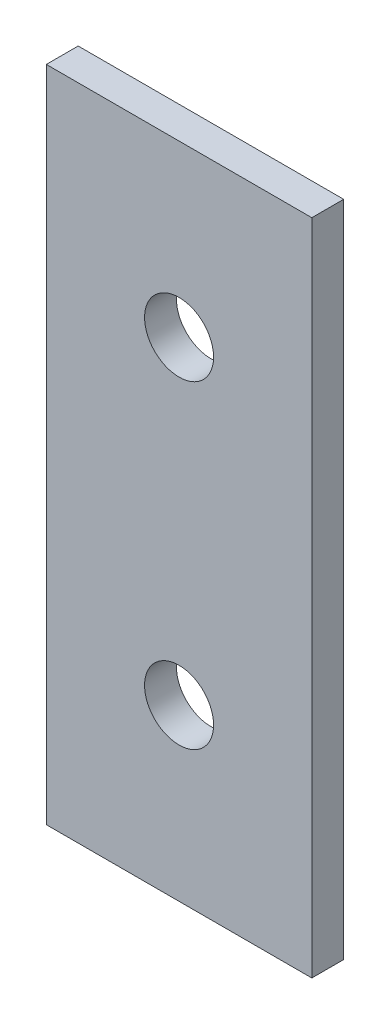
from build123d import *

# Parameters (mm, degrees)
SKETCH1_W          = 50
SKETCH1_H          = 124
EXTRUDE1_DEPTH     = 3
SKETCH2_R          = 6.5
CUT_EXTRUDE1_DEPTH = 22


with BuildPart() as part:
    # Sketch1 → Extrude1 (new, symmetric)
    with BuildSketch(Plane.XY):
        Rectangle(SKETCH1_W, SKETCH1_H)
    extrude(amount=EXTRUDE1_DEPTH, both=True)

    # Sketch2 → Cut-Extrude1 (cut)
    with BuildSketch(Plane.XY.offset(3)):
        with Locations((0, 30)):
            Circle(SKETCH2_R)
        with Locations((0, -30)):
            Circle(SKETCH2_R)
    extrude(amount=-CUT_EXTRUDE1_DEPTH, mode=Mode.SUBTRACT)


solid = part.part
